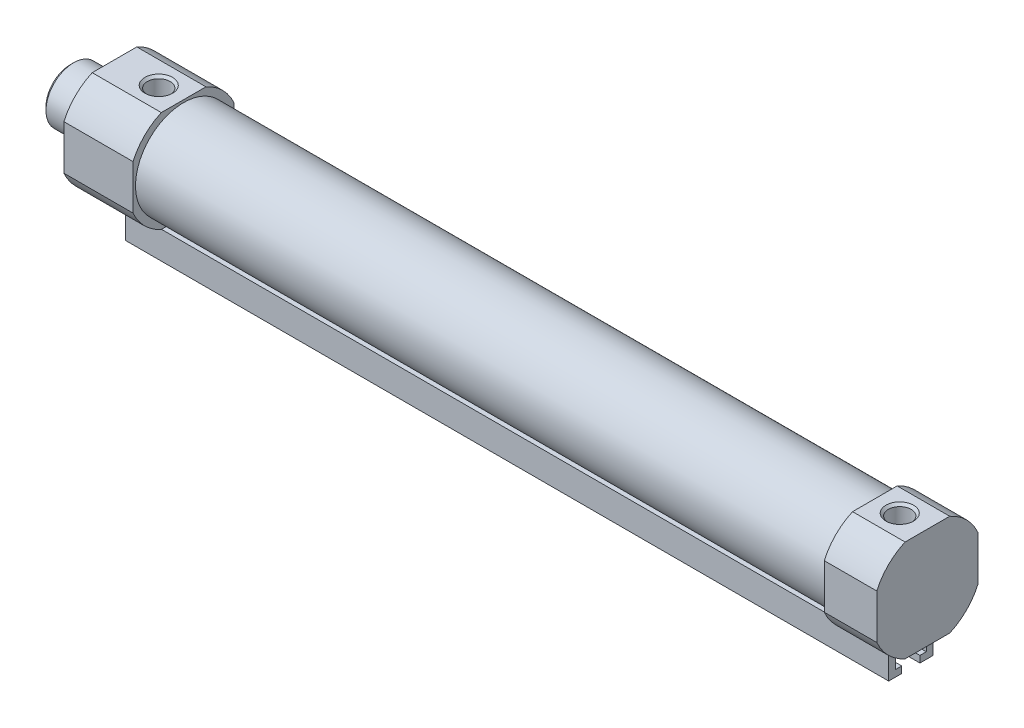
from build123d import *

# Parameters (mm, degrees)
BOSS_EXTRUDE1_DEPTH   = 12.5
SKETCH3_R             = 8.7
BOSS_EXTRUDE2_DEPTH   = 125
BOSS_EXTRUDE3_DEPTH   = 9.5
HOLE1_D               = 4.134
HOLE1_DEPTH           = 5
HOLE1_CSINK_D         = 5
HOLE1_CSINK_ANGLE     = 90
HOLE1_TIP             = 1.193383006
HOLE2_D               = 4.134
HOLE2_DEPTH           = 5
HOLE2_CSINK_D         = 5
HOLE2_CSINK_ANGLE     = 90
HOLE2_TIP             = 1.193383006
BOSS_EXTRUDE4_DEPTH   = 138
LINEAR_PATTERN1_COUNT = 2
LINEAR_PATTERN1_PITCH = 132


with BuildPart() as part:
    # Sketch1 → Revolve1 (revolve)
    with BuildSketch(Plane.XY, mode=Mode.PRIVATE) as revolve1_sk:
        Polygon((-8, 0), (-8, 4.3865), (-7.3865, 5), (0, 5), (0, 0), align=None)
    revolve(revolve1_sk.sketch.rotate(Axis((0, 0, 0), (-1, 0, 0)), 270), axis=Axis((0, 0, 0), (-1, 0, 0)))

    # Sketch2 → Boss-Extrude1 (add)
    with BuildSketch(Plane(origin=(0, 0, 0), x_dir=(0, 0, -1), z_dir=(1, 0, 0))):
        with BuildLine():
            Line((-4.034538387, -9.15), (4.034538387, -9.15))
            ThreePointArc((4.034538387, -9.15), (7.071067812, -7.071067812), (9.15, -4.034538387))
            Line((9.15, -4.034538387), (9.15, 4.034538387))
            ThreePointArc((9.15, 4.034538387), (7.071067812, 7.071067812), (4.034538387, 9.15))
            Line((4.034538387, 9.15), (-4.034538387, 9.15))
            ThreePointArc((-4.034538387, 9.15), (-7.071067812, 7.071067812), (-9.15, 4.034538387))
            Line((-9.15, 4.034538387), (-9.15, -4.034538387))
            ThreePointArc((-9.15, -4.034538387), (-7.071067812, -7.071067812), (-4.034538387, -9.15))
        make_face()
    extrude(amount=BOSS_EXTRUDE1_DEPTH)

    # Sketch3 → Boss-Extrude2 (add)
    with BuildSketch(Plane(origin=(12.5, 0, 0), x_dir=(0, 0, -1), z_dir=(1, 0, 0))):
        Circle(SKETCH3_R)
    extrude(amount=BOSS_EXTRUDE2_DEPTH)

    # Sketch4 → Boss-Extrude3 (add)
    with BuildSketch(Plane(origin=(137.5, 0, 0), x_dir=(0, 0, -1), z_dir=(1, 0, 0))):
        with BuildLine():
            Line((-4.034538387, -9.15), (4.034538387, -9.15))
            ThreePointArc((4.034538387, -9.15), (7.071067812, -7.071067812), (9.15, -4.034538387))
            Line((9.15, -4.034538387), (9.15, 4.034538387))
            ThreePointArc((9.15, 4.034538387), (7.071067812, 7.071067812), (4.034538387, 9.15))
            Line((4.034538387, 9.15), (-4.034538387, 9.15))
            ThreePointArc((-4.034538387, 9.15), (-7.071067812, 7.071067812), (-9.15, 4.034538387))
            Line((-9.15, 4.034538387), (-9.15, -4.034538387))
            ThreePointArc((-9.15, -4.034538387), (-7.071067812, -7.071067812), (-4.034538387, -9.15))
        make_face()
    extrude(amount=BOSS_EXTRUDE3_DEPTH)

    # Hole1
    with Locations(Plane(origin=(0, 9.15, 0), x_dir=(1, 0, 0), z_dir=(0, 1, 0))):
        with Locations((8, 0)):
            CounterSinkHole(HOLE1_D / 2, HOLE1_CSINK_D / 2, depth=HOLE1_DEPTH, counter_sink_angle=HOLE1_CSINK_ANGLE)
            with Locations((0, 0, -(HOLE1_DEPTH + HOLE1_TIP / 2))):  # 120° drill point
                Cone(0, HOLE1_D / 2, HOLE1_TIP, mode=Mode.SUBTRACT)

    # Hole2
    with Locations(Plane(origin=(0, 9.15, 0), x_dir=(1, 0, 0), z_dir=(0, 1, 0))):
        with Locations((142, 0)):
            CounterSinkHole(HOLE2_D / 2, HOLE2_CSINK_D / 2, depth=HOLE2_DEPTH, counter_sink_angle=HOLE2_CSINK_ANGLE)
            with Locations((0, 0, -(HOLE2_DEPTH + HOLE2_TIP / 2))):  # 120° drill point
                Cone(0, HOLE2_D / 2, HOLE2_TIP, mode=Mode.SUBTRACT)

    # Sketch9 → Cut-Revolve1 (revolve, cut)
    with BuildSketch(Plane.XY, mode=Mode.PRIVATE) as cut_revolve1_sk:
        Polygon((-8, 0), (-8, 2.5), (12.5, 2.5), (12.5, 8), (117.5, 8), (117.5, 0), align=None)
    revolve(cut_revolve1_sk.sketch.rotate(Axis((50, 0, 0), (-1, 0, 0)), 270), axis=Axis((50, 0, 0), (-1, 0, 0)), mode=Mode.SUBTRACT)

    # Sketch10 → Boss-Extrude4 (add)
    with BuildSketch(Plane(origin=(6, 0, 0), x_dir=(0, 0, -1), z_dir=(1, 0, 0))):
        Polygon((-4, -9.15), (-4, -14.15), (-1.65, -14.15), (-1.65, -12.95), (-2.8, -12.95), (-2.8, -10.35), (2.8, -10.35), (2.8, -12.95), (1.65, -12.95), (1.65, -14.15), (4, -14.15), (4, -9.15), align=None)
    extrude(amount=BOSS_EXTRUDE4_DEPTH)

    # Sketch11 → Revolve2 (revolve)
    with BuildSketch(Plane.XY):
        with BuildLine():
            Line((6.249727286, -10.35), (9, -10.35))
            Line((9, -10.35), (9, -12.35))
            ThreePointArc((9, -12.35), (7.299705908, -11.797136224), (6.249727286, -10.35))
        make_face()
    revolve2 = revolve(axis=Axis((9, 50, 0), (0, -1, 0)))

    # Linear pattern1: Revolve2 ×2
    with Locations(*[(i * LINEAR_PATTERN1_PITCH, 0, 0) for i in range(1, LINEAR_PATTERN1_COUNT)]):
        add(revolve2)


solid = part.part
